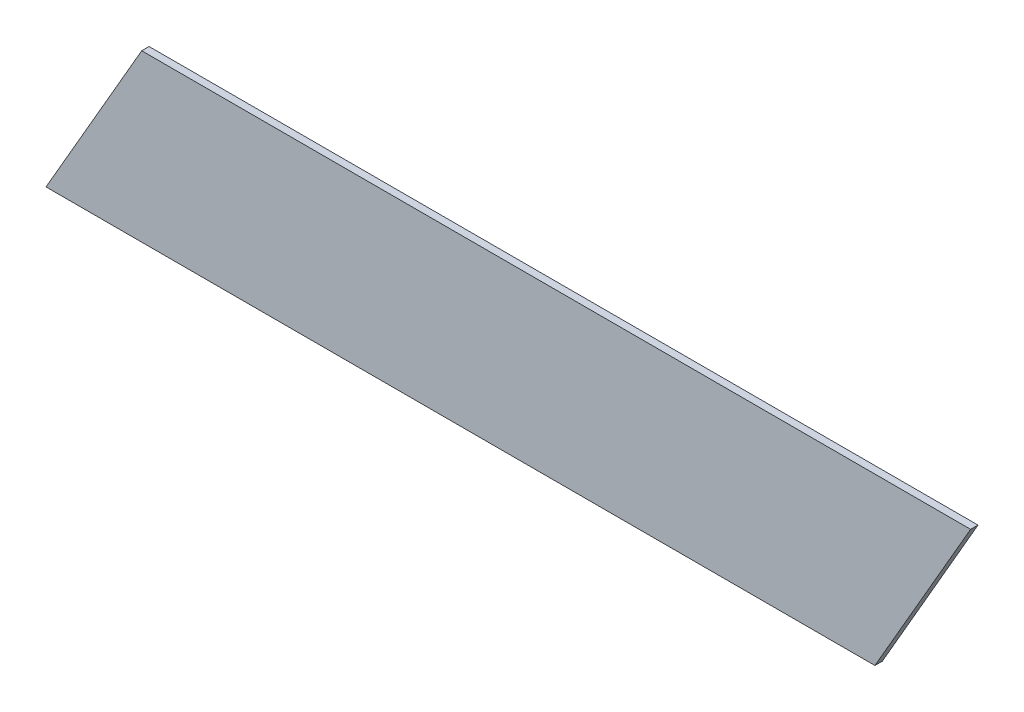
SolidWorks part; units mm, degrees
ref_plane "Front Plane" through (0, 0, 0) normal (0, 0, 1) x (1, 0, 0)
ref_plane "Top Plane" through (0, 0, 0) normal (0, 1, 0) x (1, 0, 0)
ref_plane "Right Plane" through (0, 0, 0) normal (1, 0, 0) x (0, 0, -1)
sketch "Sketch1" plane through (0, 0, 0) normal (0, 0, 1) x (1, 0, 0)
  line L0 (0, 0) -> (45, 0)
  line L1 (0, 0) -> (5.1962, 9)
  line L2 (45, 0) -> (50.1962, 9)
  line L3 (5.1962, 9) -> (50.1962, 9)
  dimension "D1" = 9
  dimension "D2" = 45
  dimension "D3" = 60
extrude "Boss-Extrude1" add sketch "Sketch1" along normal blind 0.4
